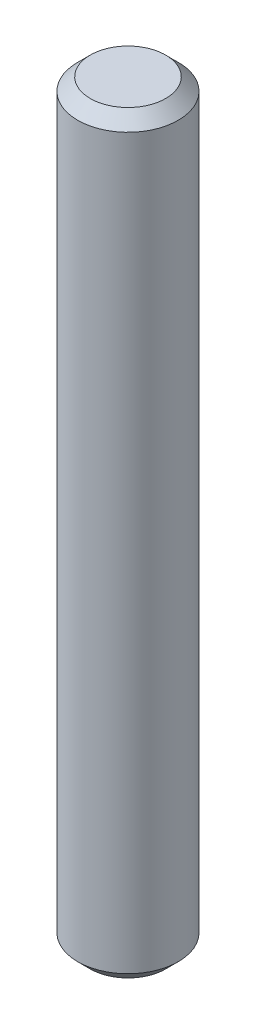
SolidWorks part; units mm, degrees
ref_plane "Front Plane" through (0, 0, 0) normal (0, 0, 1) x (1, 0, 0)
ref_plane "Top Plane" through (0, 0, 0) normal (0, 1, 0) x (1, 0, 0)
ref_plane "Right Plane" through (0, 0, 0) normal (1, 0, 0) x (0, 0, -1)
sketch "Sketch1" plane through (0, 0, 0) normal (0, 1, 0) x (1, 0, 0)
  circle A0 centre (0, 0) radius 2
  dimension "D1" = 4
extrude "Boss-Extrude1" add sketch "Sketch1" against normal blind 30
chamfer "Chamfer1" distance 0.5 angle 45 2 edges at (0, -30, 2) (0, 0, 2)
